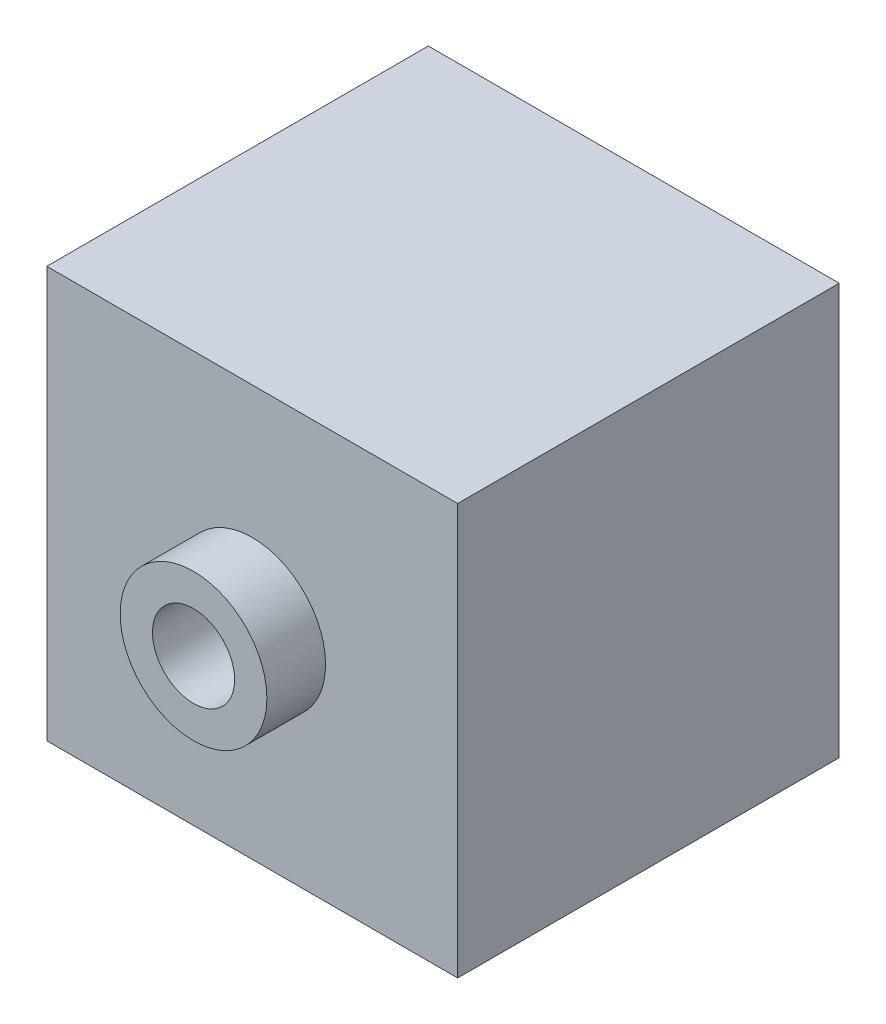
from build123d import *

# Parameters (mm, degrees)
SKETCH1_W              = 70
SKETCH1_H              = 70
BOSS_EXTRUDE1_DEPTH    = 65
SKETCH2_R              = 12.5
BOSS_EXTRUDE2_DEPTH    = 10
M16_TAPPED_HOLE1_D     = 14
M16_TAPPED_HOLE1_DEPTH = 42
M16_TAPPED_HOLE1_TIP   = 4.206024333


with BuildPart() as part:
    # Sketch1 → Boss-Extrude1 (new body)
    with BuildSketch(Plane.XY):
        Rectangle(SKETCH1_W, SKETCH1_H)
    extrude(amount=BOSS_EXTRUDE1_DEPTH)

    # Sketch2 → Boss-Extrude2 (add)
    with BuildSketch(Plane.XY.offset(65)):
        Circle(SKETCH2_R)
    extrude(amount=BOSS_EXTRUDE2_DEPTH)

    # M16 Tapped Hole1
    with Locations(Plane.XY.offset(75)):
        with Locations((0, 0)):
            Hole(M16_TAPPED_HOLE1_D / 2, depth=M16_TAPPED_HOLE1_DEPTH)
            with Locations((0, 0, -(M16_TAPPED_HOLE1_DEPTH + M16_TAPPED_HOLE1_TIP / 2))):  # 118° drill point
                Cone(0, M16_TAPPED_HOLE1_D / 2, M16_TAPPED_HOLE1_TIP, mode=Mode.SUBTRACT)


solid = part.part
